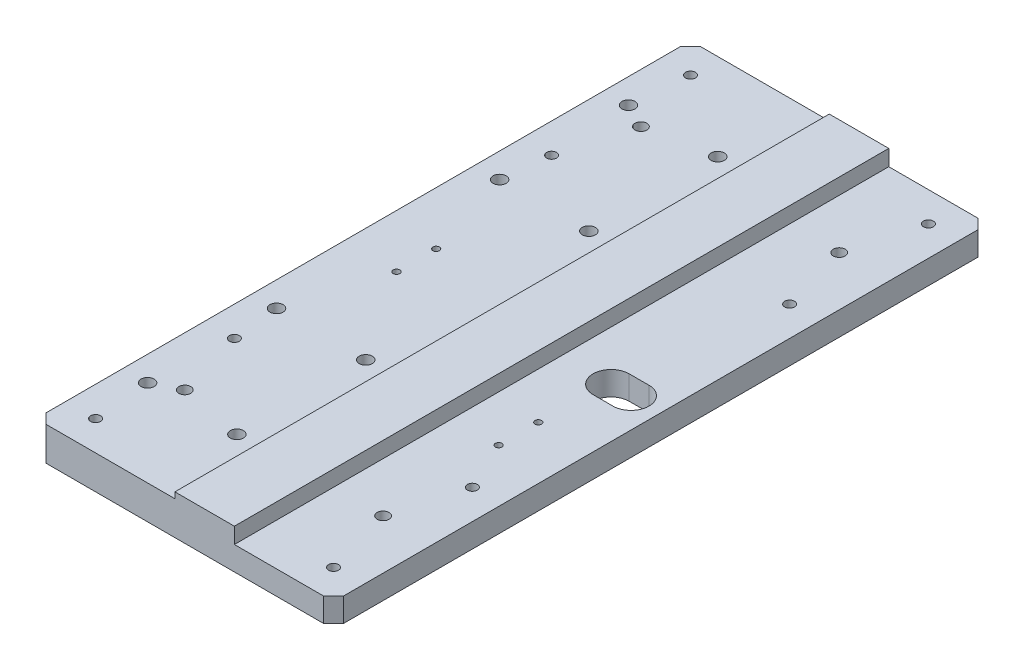
SolidWorks part; units mm, degrees
material "6061"
ref_plane "前视基准面" through (0, 0, 0) normal (0, 0, 1) x (1, 0, 0)
ref_plane "上视基准面" through (0, 0, 0) normal (0, 1, 0) x (1, 0, 0)
ref_plane "右视基准面" through (0, 0, 0) normal (1, 0, 0) x (0, 0, -1)
sketch "草图1" plane through (0, 0, 0) normal (0, 1, 0) x (1, 0, 0)
  line L1 (75, -165) -> (-75, -165)
  line L2 (75, -165) -> (75, 165)
  line L3 (75, 165) -> (-75, 165)
  line L4 (-75, -165) -> (-75, 165)
  line L5 (75, -165) -> (-75, 165) construction
  line L6 (75, 165) -> (-75, -165) construction
  point P0 (0, 0)
  dimension "D1" = 150
  dimension "D2" = 330
extrude "凸台-拉伸1" add sketch "草图1" along normal mid plane 20
sketch "草图2" plane through (0, 10, 0) normal (0, 1, 0) x (1, 0, 0)
  line L0 (75, 165) -> (-75, 165) construction
  line L1 (-75, -165) -> (-5, -165)
  line L2 (-75, -165) -> (-75, 165)
  line L3 (-75, 165) -> (-5, 165)
  line L4 (-5, -165) -> (-5, 165)
  dimension "D1" = 70
extrude "切除-拉伸1" cut sketch "草图2" against normal blind 3
sketch "草图3" plane through (0, 10, 0) normal (0, 1, 0) x (1, 0, 0)
  line L0 (75, 165) -> (-5, 165) construction
  line L1 (75, -165) -> (25, -165)
  line L2 (75, -165) -> (75, 165)
  line L3 (75, 165) -> (25, 165)
  line L4 (25, -165) -> (25, 165)
  dimension "D1" = 50
extrude "切除-拉伸2" cut sketch "草图3" against normal blind 8
hole_wizard "大小mm 暗销孔1" positions "草图4" profile "草图5" hole size "Ø1.0" standard "ISO" end condition through all
sketch "草图4" plane through (0, 7, 0) normal (0, 1, 0) x (1, 0, 0)
  point P0 (-62.5, 121.25)
  point P3 (-17.5, 121.25)
  point P6 (-62.5, 56.25)
  point P9 (-17.5, 56.25)
  point P12 (-62.5, -56.25)
  point P15 (-17.5, -56.25)
  point P18 (-62.5, -121.25)
  point P21 (-17.5, -121.25)
sketch "草图5" plane through (-62.5, 7, -121.25) normal (1, 0, 0) x (0, 0, 1)
  line L0 (0, 0) -> (0, 17)
  line L1 (0, 17) -> (0.5, 17)
  line L2 (0.5, 17) -> (0.5, 0)
  line L5 (0.5, 0) -> (0, 0)
  line L11 (0, -6.35) -> (0, 107.95) construction
  dimension "通孔孔直径" = 1
  dimension "通孔孔深度" = 17
hole_wizard "M6 六角凹头螺钉的柱形沉头孔1" positions "草图6" profile "草图7" counterbore size "M6" standard "ISO" end condition through all
sketch "草图6" plane through (0, -10, 0) normal (0, -1, 0) x (-1, 0, 0)
  point P0 (17.5, 121.25)
  point P3 (62.5, 121.25)
  point P6 (17.5, 56.25)
  point P9 (62.5, 56.25)
  point P12 (17.5, -56.25)
  point P15 (62.5, -56.25)
  point P18 (17.5, -121.25)
  point P21 (62.5, -121.25)
sketch "草图7" plane through (-17.5, -10, -121.25) normal (1, 0, 0) x (0, 0, -1)
  line L0 (0, 0) -> (0, 20)
  line L1 (0, 20) -> (3.3, 20)
  line L3 (3.3, 20) -> (3.3, 8)
  line L4 (3.3, 8) -> (5.5, 8)
  line L5 (5.5, 8) -> (5.5, 0)
  line L7 (5.5, 0) -> (0, 0)
  line L11 (0, -6.35) -> (0, 107.95) construction
  dimension "通孔孔直径" = 6.6
  dimension "通孔孔深度" = 20
  dimension "柱形沉头孔直径" = 11
  dimension "柱形沉头孔深度" = 8
hole_wizard "大小mm 暗销孔0" positions "草图10" profile "草图11" hole size "Ø6.0" standard "ISO" end condition through all
sketch "草图10" plane through (0, -10, 0) normal (0, -1, 0) x (-1, 0, 0)
  line L0 (44.5, 115) -> (55.5, 115) construction
  line L1 (44.5, -115) -> (55.5, -115) construction
  arc A0 (47.5, 118) -> (47.5, 112) centre (47.5, 115) ccw construction
  arc A1 (52.5, 112) -> (52.5, 118) centre (52.5, 115) ccw construction
  arc A2 (47.5, -112) -> (47.5, -118) centre (47.5, -115) ccw construction
  arc A3 (52.5, -118) -> (52.5, -112) centre (52.5, -115) ccw construction
  point P3 (-50, 115)
  point P9 (-50, -115)
  point P25 (50, 115)
  point P38 (50, -115)
sketch "草图11" plane through (50, -10, -115) normal (1, 0, 0) x (0, 0, -1)
  line L0 (0, 0) -> (0, 20)
  line L1 (0, 20) -> (3, 20)
  line L2 (3, 20) -> (3, 0)
  line L5 (3, 0) -> (0, 0)
  line L11 (0, -6.35) -> (0, 107.95) construction
  dimension "通孔孔直径" = 6
  dimension "通孔孔深度" = 20
hole_wizard "M6 螺纹孔1" positions "草图12" profile "草图13" tap size "M6" standard "ISO" end condition through all
sketch "草图12" plane through (0, -10, 0) normal (0, -1, 0) x (-1, 0, 0)
  point P0 (60, -150)
  point P3 (-60, -150)
  point P6 (-60, -80)
  point P9 (60, -80)
  point P12 (60, 80)
  point P15 (60, 150)
  point P18 (-60, 150)
  point P21 (-60, 80)
sketch "草图13" plane through (-60, -10, 150) normal (1, 0, 0) x (0, 0, -1)
  line L0 (0, 0) -> (0, 20)
  line L1 (0, 20) -> (2.5, 20)
  line L2 (2.5, 20) -> (2.5, 0)
  line L5 (2.5, 0) -> (0, 0)
  line L11 (0, -6.35) -> (0, 107.95) construction
  dimension "通孔螺纹孔钻头直径" = 5
  dimension "通孔螺纹孔钻头深度" = 20
cosmetic thread "孔螺蚊线1" parameters "D2"=6
cosmetic thread "孔螺蚊线2" parameters "D2"=6
cosmetic thread "孔螺蚊线3" parameters "D2"=6
cosmetic thread "孔螺蚊线4" parameters "D2"=6
cosmetic thread "孔螺蚊线5" parameters "D2"=6
cosmetic thread "孔螺蚊线6" parameters "D2"=6
cosmetic thread "孔螺蚊线7" parameters "D2"=6
cosmetic thread "孔螺蚊线8" parameters "D2"=6
chamfer "倒角1" distance 5 angle 45 4 edges at (-75, -1.5, 165) (-75, -1.5, -165) (75, -4, -165) (75, -4, 165)
sketch "草图14" plane through (0, -10, 0) normal (0, -1, 0) x (1, 0, 0)
  line L0 (-75, 0) -> (89.1737, 0) construction
  line L1 (-75, -160) -> (-75, 160) construction
  line L2 (50, 0) -> (60, 0) construction
  line L3 (50, 9.1) -> (60, 9.1)
  line L4 (50, -9.1) -> (60, -9.1)
  line L5 (55, -165) -> (55, 182.901) construction
  line L6 (70, -165) -> (-70, -165) construction
  line L7 (75, 160) -> (75, -160) construction
  arc A0 (50, 9.1) -> (50, -9.1) centre (50, 0) ccw
  arc A1 (60, -9.1) -> (60, 9.1) centre (60, 0) ccw
  point P7 (55, 0)
  dimension "D1" = 9.1
  dimension "D2" = 20
  dimension "D3" = 10
extrude "切除-拉伸3" cut sketch "草图14" against normal through all
hole_wizard "M4 螺纹孔1" positions "草图17" profile "草图18" tap size "M4" standard "ISO" end condition through all
sketch "草图17" plane through (0, -10, 0) normal (0, -1, 0) x (-1, 0, 0)
  line L0 (60.75, 10) -> (35.75, 10) construction
  line L2 (60.75, -10) -> (35.75, -10) construction
  line L4 (-35.75, -55) -> (-60.75, -55) construction
  line L6 (-35.75, -35) -> (-60.75, -35) construction
  arc A0 (58.25, 7.5) -> (58.25, 12.5) centre (58.25, 10) ccw construction
  arc A1 (38.25, 12.5) -> (38.25, 7.5) centre (38.25, 10) ccw construction
  arc A2 (58.25, -12.5) -> (58.25, -7.5) centre (58.25, -10) ccw construction
  arc A3 (38.25, -7.5) -> (38.25, -12.5) centre (38.25, -10) ccw construction
  arc A4 (-38.25, -57.5) -> (-38.25, -52.5) centre (-38.25, -55) ccw construction
  arc A5 (-58.25, -52.5) -> (-58.25, -57.5) centre (-58.25, -55) ccw construction
  arc A6 (-38.25, -37.5) -> (-38.25, -32.5) centre (-38.25, -35) ccw construction
  arc A7 (-58.25, -32.5) -> (-58.25, -37.5) centre (-58.25, -35) ccw construction
  point P0 (-48.25, -35)
  point P2 (-48.25, -55)
  point P4 (48.25, -10)
  point P6 (48.25, 10)
sketch "草图18" plane through (48.25, -10, 35) normal (1, 0, 0) x (0, 0, -1)
  line L0 (0, 0) -> (0, 20)
  line L1 (0, 20) -> (1.65, 20)
  line L2 (1.65, 20) -> (1.65, 0)
  line L5 (1.65, 0) -> (0, 0)
  line L11 (0, -6.35) -> (0, 107.95) construction
  dimension "通孔螺纹孔钻头直径" = 3.3
  dimension "通孔螺纹孔钻头深度" = 20
cosmetic thread "孔螺蚊线9" parameters "D2"=4
cosmetic thread "孔螺蚊线10" parameters "D2"=4
cosmetic thread "孔螺蚊线11" parameters "D2"=4
cosmetic thread "孔螺蚊线12" parameters "D2"=4
